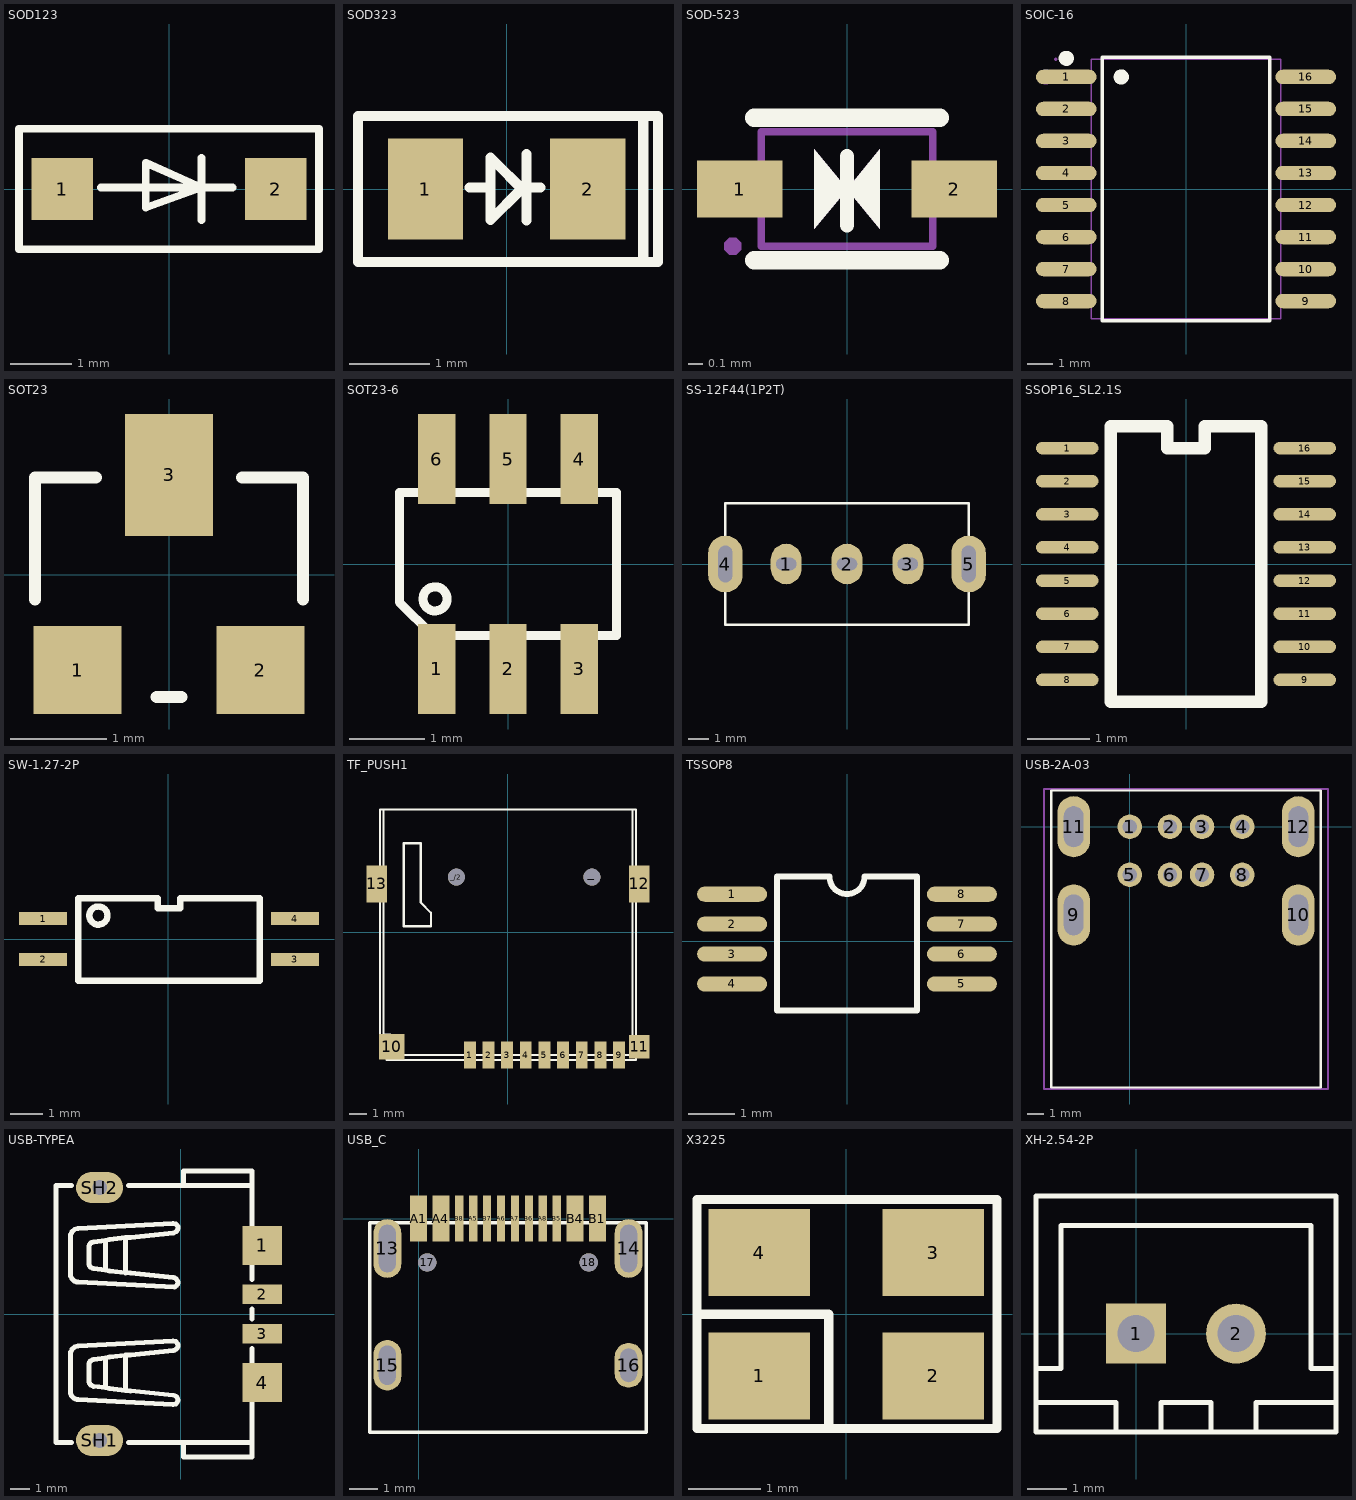
[diagram p0: the footprints below, top view; thin cyan lines are the x and y axes]
# Altium footprint library MISC82162-2.PcbLib: 66 footprints (part 4 of 5)
Each footprint in its own frame and in the unit in brackets; x right, y up, seen from the top. Pads: shape width x height; smd on the part's side, far side on the other; paste and mask are expansions set on the pad; w line width, h text height; cw(c..) or ccw(c..) is an arc to the next point about the centre after c.

## SOD123 [mil]
pads (2):
  rrect0% 40x40 smd: 1(-69,0) 2(69,0)
Top Overlay:
  lines w5: -44,1 41,1 ; 21,-20 21,20 ; -97,-39 97,-39 97,39 -97,39 -97,-39 ; -15,-12 21,1 -15,17 -15,-12

## SOD323 [mil]
pads (2):
  rect 37x50 smd: 1(-40,0) 2(40,0)
Top Overlay:
  lines w5: -18.14,0.79 -8.29,0.79 ; 6.78,-0.54 -7.95,-15.27 -7.95,15.56 9.77,-2.15 ; 9.84,-15.53 9.84,17.11 ; 9.88,0.79 16.65,0.79 ; 67.37,-34.65 67.37,35.13 ; 74.57,35.91 74.57,-35.94 -73.22,-35.94 -73.22,35.94 74.63,35.94

## SOD-523 [mm]
pads (2):
  rect 0.6x0.4 smd: 1(-0.75,0) 2(0.75,0)
Top Overlay:
  region: 0,0 0.229,0.279 0.229,-0.279
  region: 0,0 -0.229,-0.279 -0.229,0.279
  lines w0.1: 0,-0.254 0,0.229
  lines w0.13: -0.65,-0.5 0.65,-0.5 ; -0.65,0.5 0.65,0.5
Mechanical 6:
  region: -0.229,0.279 -0.229,-0.279 0,0
  region: 0.229,0.279 0.229,-0.279 0,0
Mechanical 15:
  region: -0.74,-0.4 -0.74,-0.375 -0.775,-0.34 -0.825,-0.34 -0.86,-0.375 -0.86,-0.4 -0.86,-0.425 -0.825,-0.46 -0.775,-0.46 -0.74,-0.425
  region: 0.8,-0.152 0.463,-0.152 0.463,0.148 0.8,0.148
  region: -0.8,0.15 -0.463,0.15 -0.463,-0.15 -0.8,-0.15
  lines w0.051: -0.6,-0.4 -0.6,0.4 0.6,0.4 0.6,-0.4 -0.6,-0.4

## SOIC-16 [mm]
pads (16):
  oval 2.401x0.574 smd: 1(-4.75,4.445) 2(-4.75,3.175) 3(-4.75,1.905) 4(-4.75,0.635) 5(-4.75,-0.635) 6(-4.75,-1.905) 7(-4.75,-3.175) 8(-4.75,-4.445) 9(4.75,-4.445) 10(4.75,-3.175) 11(4.75,-1.905) 12(4.75,-0.635) 13(4.75,0.635) 14(4.75,1.905) 15(4.75,3.175) 16(4.75,4.445)
Top Overlay:
  circle w0.3: c-2.569,4.445 r0.15
  circle w0.3: c-4.75,5.184 r0.15
  lines w0.152: -3.321,-5.226 3.321,-5.226 3.321,5.226 -3.321,5.226 -3.321,-5.226
Mechanical 6:
  circle w0.3: c-5.563,4.445 r0.15
Mechanical 15:
  drawing of 37 lines, arcs and shapes, not listed

## SOT23 [mil]
pads (3):
  rect 36x36 smd: 1(-37.5,-39) 2(37.5,-39)
  rect 36x50 smd: 3(0,41)
Top Overlay:
  lines w5: -55,-10 -55,40 -30,40 ; -5,-50 5,-50 ; 30,40 55,40 55,-10

## SOT23-6 [mm]
pads (6):
  rect 0.5x1.2 smd: 1(-0.95,-1.4) 2(0,-1.4) 3(0.95,-1.4) 4(0.95,1.4) 5(0,1.4) 6(-0.95,1.4)
Top Overlay:
  circle w0.12: c-0.974,-0.466 r0.161
  lines w0.12: -1.45,-0.508 -1.006,-0.952 -1.006,-0.95 1.45,-0.95 1.45,0.95 -1.45,0.95 -1.45,-0.508

## SS-12F44(1P2T) [mm]
pads (5):
  oval 1.524x2 hole 0.6 slot 1 at 0 deg: 1(-3,0) 2(0,0) 3(3,0)
  oval 1.7x2.8 hole 0.7 slot 1.8 at 90 deg: 4(-6,0) 5(6,0)
Top Overlay:
  lines w0.127: -6,-3 -6,3 6,3 6,-3 -6,-3

## SSOP16_SL2.1S [mm]
height 1.27
pads (16):
  oval 1x0.2 smd: 1(-1.9,1.855) 2(-1.9,1.325) 3(-1.9,0.795) 4(-1.9,0.265) 5(-1.9,-0.265) 6(-1.9,-0.795) 7(-1.9,-1.325) 8(-1.9,-1.855) 9(1.9,-1.855) 10(1.9,-1.325) 11(1.9,-0.795) 12(1.9,-0.265) 13(1.9,0.265) 14(1.9,0.795) 15(1.9,1.325) 16(1.9,1.855)
Top Overlay:
  lines w0.2: -1.2,-2.2 -1.2,2.2 -0.3,2.2 -0.3,1.855 0.3,1.855 0.3,2.2 1.2,2.2 1.2,-2.2 -1.2,-2.2

## SW-1.27-2P [mm]
height 2.65
pads (4):
  rect 1.5x0.4 smd: 1(-3.9,0.65)
  rect 1.5x0.4 smd paste-0.05: 2(-3.9,-0.62) 3(3.95,-0.62) 4(3.95,0.65)
Top Overlay:
  circle w0.2: c-2.175,0.745 r0.283
  lines w0.2: -2.8,-1.285 -2.8,1.285 -0.328,1.285 -0.328,0.968 0.378,0.968 0.378,1.285 2.85,1.285 2.85,-1.285 -2.8,-1.285

## TF_PUSH1 [mm]
pads (15):
  rect 0.7x1.6 smd: 1(-2.25,-7.25) 2(-1.15,-7.25) 3(-0.05,-7.25) 4(1.05,-7.25) 5(2.15,-7.25) 6(3.25,-7.25) 7(4.35,-7.25) 8(5.45,-7.25) 9(6.55,-7.25)
  rrect0% 1.5x1.5 smd: 10(-6.85,-6.75)
  rect 1.2x1.4 smd: 11(7.75,-6.75)
  rect 1.2x2.2 smd: 12(7.75,2.85) 13(-7.75,2.85)
  round 1 hole 1: _(4.95,3.25) _/2(-3.05,3.25)
Top Overlay:
  lines w0.127: -7.35,7.25 7.35,7.25 ; -7.35,7.25 -7.55,7.25 -7.55,-6.25 -7.15,-6.25 -7.15,-7.53 7.55,-7.53 7.55,7.25 7.35,7.25 ; -7.35,7.25 -7.35,-6.05 -6.95,-6.05 -6.95,-7.25 7.35,-7.25 7.35,7.25 ; -6.15,0.35 -6.15,5.25 -5.15,5.25 -5.15,1.75 -4.55,1.15 -4.55,0.35 -6.15,0.35

## TSSOP8 [mil]
pads (8):
  oval 60x13 smd: 1(-98.43,40.4) 2(-98.43,14.8) 3(-98.43,-10.8) 4(-98.43,-36.4) 5(98.43,-36.4) 6(98.43,-10.8) 7(98.43,14.8) 8(98.43,40.4)
Top Overlay:
  lines w5: -60,-59.06 60,-59.06 60,55.51 15,55.51 cw(c0,55.51) -15,55.51 -60,55.51 -60,-59.06

## USB-2A-03 [mil]
pads (12):
  round 60 hole 35: 1(0,0) 2(98.43,0) 3(177.17,0) 4(275.59,0) 5(0,-118.11) 6(98.43,-118.11) 7(177.17,-118.11) 8(275.59,-118.11)
  oval 80x150 hole 48 slot 100 at 90 deg: 9(-137.8,-216.54) 10(413.39,-216.54) 11(-137.8,0) 12(413.39,0)
Top Overlay:
  lines w5: -192.91,-639.76 -192.91,88.58 ; -192.91,-639.76 468.5,-639.76 ; -192.91,-639.76 -192.91,88.58 ; -192.91,-639.76 468.5,-639.76 ; -192.91,88.58 468.5,88.58 ; -192.91,88.58 468.5,88.58 ; 468.5,-639.76 468.5,88.58 ; 468.5,-639.76 468.5,88.58
Mechanical 20:
  lines w5: -210.63,-643.7 -210.63,92.52 486.22,92.52 486.22,-643.7 -210.63,-643.7

## USB-TYPEA [mm]
pads (6):
  rect 2x2 smd: 1(4.15,3.5) 4(4.15,-3.5)
  rect 2x1 smd: 2(4.15,1) 3(4.15,-1)
  oval 2.4x1.6 hole 0.75: SH1(-4.15,-6.45) SH2(-4.15,6.45)
Top Overlay:
  lines w0.254: -5.572,-6.544 -6.372,-6.544 -6.372,6.545 -5.572,6.545 ; -5.26,1.628 -5.332,1.642 -5.392,1.662 -5.445,1.69 -5.496,1.727 -5.533,1.765 -5.571,1.818 -5.602,1.88 -5.624,1.945 -5.624,4.05 -5.548,4.209 -5.419,4.321 -5.254,4.368 -0.406,4.621 -0.265,4.58 ; -5.259,-4.368 -5.315,-4.361 -5.374,-4.343 -5.43,-4.315 -5.485,-4.276 -5.534,-4.228 -5.572,-4.178 -5.603,-4.119 -5.624,-4.056 -5.624,-1.944 -5.548,-1.785 -5.419,-1.674 -5.254,-1.626 -0.406,-1.373 -0.265,-1.415 ; -5.254,-4.368 -0.406,-4.621 -0.265,-4.585 -0.171,-4.468 -0.153,-4.397 -0.165,-4.321 -0.242,-4.197 -0.377,-4.144 -2.583,-3.915 -2.83,-3.891 ; -5.254,1.627 -0.336,1.38 -0.28,1.406 -0.229,1.444 -0.195,1.483 -0.169,1.531 -0.156,1.58 -0.155,1.631 -0.168,1.684 -0.192,1.734 ; -2.676,-6.544 3.624,-6.544 ; -2.676,6.545 3.624,6.545 ; -0.261,-1.417 -0.223,-1.451 -0.191,-1.489 -0.171,-1.525 -0.157,-1.567 -0.154,-1.604 -0.159,-1.65 -0.173,-1.698 -0.195,-1.744 -0.242,-1.797 -0.306,-1.838 -0.377,-1.856 -2.583,-2.085 -2.83,-2.103 ; -0.261,4.577 -0.216,4.537 -0.185,4.497 -0.164,4.451 -0.154,4.4 -0.157,4.351 -0.173,4.299 -0.201,4.247 -0.242,4.197 -0.377,4.139 -2.583,3.909 -2.83,3.892 ; -0.195,1.739 -0.242,1.798 -0.306,1.839 -0.377,1.856 -2.583,2.086 -2.83,2.103 ; 0.123,-6.544 0.123,-7.297 3.624,-7.297 3.624,-4.25 ; 0.123,6.545 0.123,7.292 3.624,7.292 3.624,4.25 ; 3.624,-2.75 3.624,-1.75 ; 3.624,-0.25 3.624,0 3.624,0.25 ; 3.624,1.75 3.624,2.75 ; -3.854,-3.756 -4.46,-3.685 -4.542,-3.656 -4.607,-3.609 -4.659,-3.544 -4.689,-3.468 -4.695,-3.386 -4.695,-2.615 -4.689,-2.532 -4.659,-2.456 -4.607,-2.391 -4.542,-2.338 -4.46,-2.315 -3.854,-2.238 ; -3.854,-3.756 -3.854,-2.238 ; -3.854,-3.756 -3.654,-3.791 -2.83,-3.891 ; -3.854,-2.238 -3.654,-2.203 -2.83,-2.103 ; -3.854,2.239 -4.46,2.315 -4.542,2.339 -4.607,2.386 -4.659,2.451 -4.689,2.527 -4.695,2.609 -4.695,3.386 -4.689,3.468 -4.659,3.544 -4.607,3.609 -4.542,3.656 -4.46,3.68 -3.854,3.756 ; -3.854,2.239 -3.854,3.756 ; -3.854,2.239 -3.654,2.203 -2.83,2.103 ; -3.854,3.756 -3.654,3.792 -2.83,3.892 ; -2.83,-3.891 -2.83,-2.103 ; -2.83,2.103 -2.83,3.892

## USB_C [mm]
pads (18):
  oval 1x2.1 hole 0.6 slot 1.7 at 90 deg: 13(-1.12,-1.07) 14(7.52,-1.07)
  oval 1x1.8 / inner oval 1x1.6 / far side oval 1x1.6 hole 0.6 slot 1.4 at 90 deg: 15(-1.12,-5.25)
  oval 1x1.6 hole 0.6 slot 1.2 at 90 deg: 16(7.52,-5.25)
  round 0.65 hole 0.65 unplated: 17(0.31,-1.57) 18(6.09,-1.57)
  rect 0.6x1.64 smd: A1(0,0) A4(0.8,0) B1(6.4,0) B4(5.6,0)
  rect 0.3x1.64 smd: A5(1.95,0) A6(2.95,0) A7(3.45,0) A8(4.45,0) B5(4.95,0) B6(3.95,0) B7(2.45,0) B8(1.45,0)
Top Overlay:
  lines w0.127: -1.75,-7.65 -1.75,-0.15 8.15,-0.15 8.15,-7.65 -1.75,-7.65
Top Paste:
  region: 8.147,-5.55 8.159,-4.95 8.111,-4.705 7.972,-4.498 7.765,-4.359 7.52,-4.311 7.275,-4.359 7.068,-4.498 6.929,-4.705 6.881,-4.95 6.893,-4.95 6.881,-5.55 6.929,-5.795 7.068,-6.002 7.275,-6.141 7.52,-6.189 7.765,-6.141 7.972,-6.002 8.111,-5.795 8.159,-5.55
  region: -0.493,-5.65 -0.481,-4.85 -0.529,-4.605 -0.668,-4.398 -0.875,-4.259 -1.12,-4.211 -1.365,-4.259 -1.572,-4.398 -1.711,-4.605 -1.759,-4.85 -1.747,-4.85 -1.759,-5.65 -1.711,-5.895 -1.572,-6.102 -1.365,-6.241 -1.12,-6.289 -0.875,-6.241 -0.668,-6.102 -0.529,-5.895 -0.481,-5.65
  region: 8.147,-1.62 8.159,-0.52 8.111,-0.275 7.972,-0.068 7.765,0.071 7.52,0.119 7.275,0.071 7.068,-0.068 6.929,-0.275 6.881,-0.52 6.893,-0.52 6.881,-1.62 6.929,-1.865 7.068,-2.072 7.275,-2.211 7.52,-2.259 7.765,-2.211 7.972,-2.072 8.111,-1.865 8.159,-1.62
  region: -0.493,-1.62 -0.481,-0.52 -0.529,-0.275 -0.668,-0.068 -0.875,0.071 -1.12,0.119 -1.365,0.071 -1.572,-0.068 -1.711,-0.275 -1.759,-0.52 -1.747,-0.52 -1.759,-1.62 -1.711,-1.865 -1.572,-2.072 -1.365,-2.211 -1.12,-2.259 -0.875,-2.211 -0.668,-2.072 -0.529,-1.865 -0.481,-1.62

## X3225 [mm]
pads (4):
  rect 1.4x1.2 smd: 1(-1.2,-0.85) 2(1.2,-0.85) 3(1.2,0.85) 4(-1.2,0.85)
Top Overlay:
  lines w0.127: -2.05,0 -0.24,0 -0.24,-1.57 ; -2.059,-1.576 2.081,-1.576 2.081,1.584 -2.059,1.584 -2.059,-1.576

## XH-2.54-2P [mil]
pads (2):
  rect 60x60 / inner round 60 / far side rect 60x60 hole 37: 1(0,0)
  round 60 hole 37: 2(100,0)
Top Overlay:
  lines w5: -100,-68.9 -20,-68.9 -20,-98.43 ; -100,-35 -75,-35 -75,108.27 175,108.27 175,-35 200,-35 ; 25,-98.43 25,-68.9 75,-68.9 75,-98.43 ; 120,-98.43 120,-68.9 200,-68.9 ; -100,-98.43 -100,137.8 200,137.8 200,-98.43 -100,-98.43
Bottom Overlay:
  region: 65,-55.83 35,-55.83 35,91.36 65,91.36